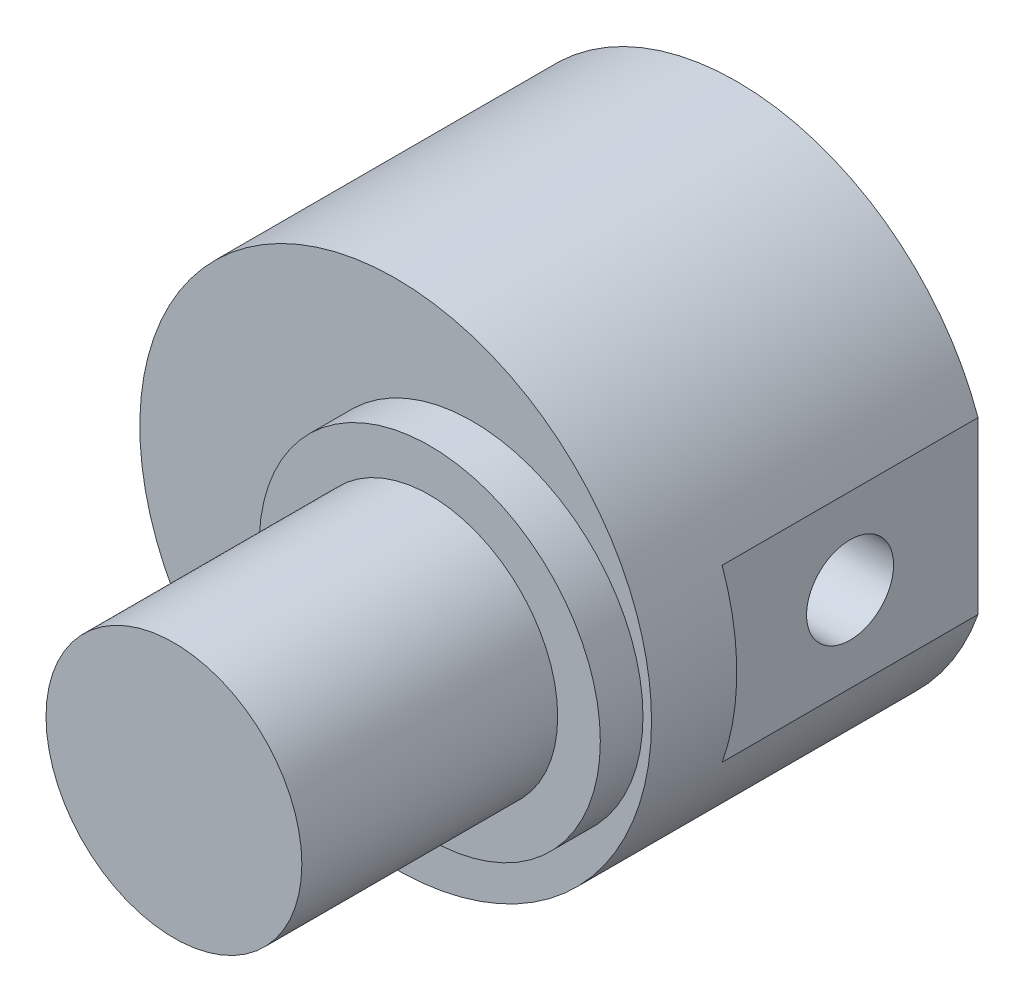
SolidWorks part; units mm, degrees
ref_plane "前视基准面" through (0, 0, 0) normal (0, 0, 1) x (1, 0, 0)
ref_plane "上视基准面" through (0, 0, 0) normal (0, 1, 0) x (1, 0, 0)
ref_plane "右视基准面" through (0, 0, 0) normal (1, 0, 0) x (0, 0, -1)
sketch "草图1" plane through (0, 0, 0) normal (0, 0, 1) x (1, 0, 0)
  circle A0 centre (0, 0) radius 30
extrude "凸台-拉伸1" add sketch "草图1" along normal blind 40
sketch "草图2" plane through (0, 0, 40) normal (0, 0, 1) x (1, 0, 0)
  circle A0 centre (9, 0) radius 20
extrude "凸台-拉伸2" add sketch "草图2" along normal blind 5
sketch "草图3" plane through (0, 0, 45) normal (0, 0, 1) x (1, 0, 0)
  circle A0 centre (9, 0) radius 15
extrude "凸台-拉伸3" add sketch "草图3" along normal blind 30
sketch "草图5" plane through (0, 0, 0) normal (0, 0, -1) x (-1, 0, 0)
  line L0 (-11.4334, 0) -> (-50.533, 0) construction
  line L2 (-30.26, 10) -> (-28.2843, 10)
  line L3 (-28.2843, 10) -> (-28.2843, -10)
  line L4 (-28.2843, -10) -> (-32.2203, -10)
  line L5 (-32.2203, -10) -> (-32.2203, 10)
  line L6 (-32.2203, 10) -> (-30.26, 10)
  circle A0 centre (0, 0) radius 18
  circle A3 centre (0, 0) radius 30 construction
extrude "切除-拉伸1" cut sketch "草图5" against normal blind 30
hole_wizard "M12 螺纹孔1" positions "草图11" profile "草图9" tap size "M12" standard "Iso"
sketch "草图11" plane through (28.2843, 0, 0) normal (1, 0, 0) x (0, 0, -1)
  line L0 (0, -10) -> (0, 10) construction
  point P0 (-15, 0)
  dimension "D1" = 15
sketch "草图9" plane through (28.2843, 0, 15) normal (0, 1, 0) x (0, 0, -1)
  line L0 (0, 0) -> (0, 32.3144)
  line L1 (0, 32.3144) -> (5.1, 29.25)
  line L2 (5.1, 29.25) -> (5.1, 0)
  line L5 (5.1, 0) -> (0, 0)
  line L10 (0, 32.3144) -> (-5.1, 29.25) construction
  line L11 (0, -6.35) -> (0, 107.95) construction
  dimension "螺纹孔钻头直径" = 10.2
  dimension "螺纹孔钻头深度" = 29.25
  dimension "导头角度" = 118
cosmetic thread "孔螺蚊线1" parameters "D1"=11.0219, "D2"=12
